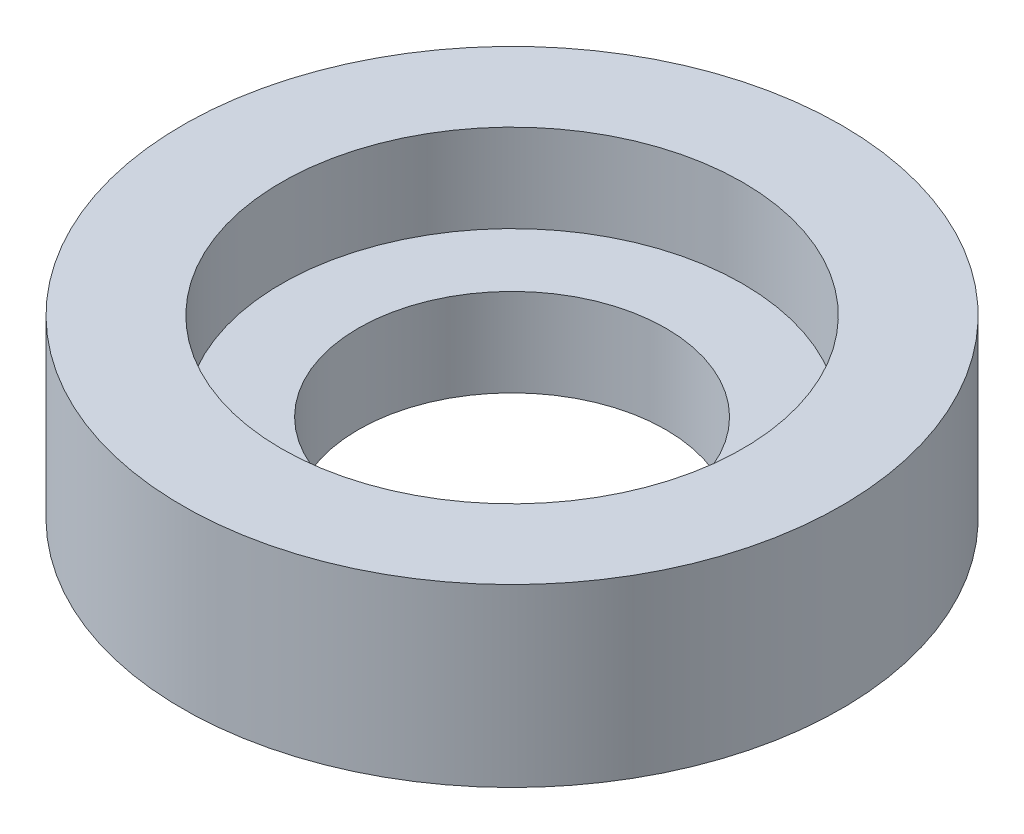
SolidWorks part; units mm, degrees
ref_plane "Front Plane" through (0, 0, 0) normal (0, 0, 1) x (1, 0, 0)
ref_plane "Top Plane" through (0, 0, 0) normal (0, 1, 0) x (1, 0, 0)
ref_plane "Right Plane" through (0, 0, 0) normal (1, 0, 0) x (0, 0, -1)
sketch "Sketch1" plane through (0, 0, 0) normal (0, 0, 1) x (1, 0, 0)
  line L0 (-3.5, 0) -> (-7.5, 0)
  line L1 (-7.5, 0) -> (-7.5, 4)
  line L2 (-7.5, 4) -> (-5.25, 4)
  line L3 (-5.25, 4) -> (-5.25, 2)
  line L4 (-5.25, 2) -> (-3.5, 2)
  line L5 (-3.5, 2) -> (-3.5, 0)
  line L6 (0, 0) -> (0, 16.9452) construction
  dimension "D1" = 3.5
  dimension "D2" = 7.5
  dimension "D3" = 5.25
  dimension "D4" = 4
  dimension "D5" = 2
revolve "Revolve1" add sketch "Sketch1" angle 360 about L6
